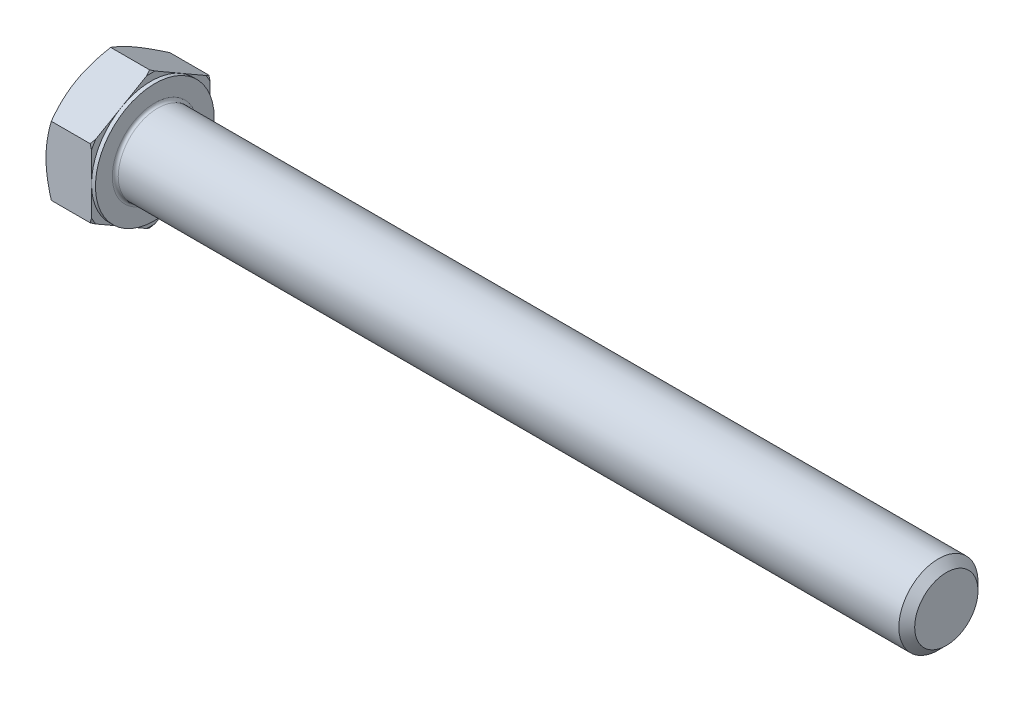
SolidWorks part; units mm, degrees
extrude "Base-Extrude" add sketch "Sketch1" along normal blind 10
sketch "Sketch1" plane through (0, 0, 0) normal (1, 0, 0) x (0, 0, -1)
  line L0 (12, 6.9282) -> (12, -6.9282)
  line L1 (-12, 6.9282) -> (-12, -6.9282)
  line L2 (12, -6.9282) -> (0, -13.8564)
  line L3 (0, -13.8564) -> (-12, -6.9282)
  line L4 (12, 6.9282) -> (0, 13.8564)
  line L5 (0, 13.8564) -> (-12, 6.9282)
revolve "Cut-Revolve1" cut sketch "Sketch3" angle 360 about L6
sketch "Sketch3" plane through (0, 0, 0) normal (0, 0, 1) x (1, 0, 0)
  line L0 (0, 12) -> (3.9585, 18.8564)
  line L1 (0, 13.8564) -> (0, 6.9282) construction
  line L2 (3.9585, 18.8564) -> (3.9585, 23.8564)
  line L3 (3.9585, 23.8564) -> (-10, 23.8564)
  line L4 (-10, 23.8564) -> (-10, 12)
  line L5 (-10, 12) -> (0, 12)
  line L6 (0, 0) -> (99.06, 0) construction
  line L7 (10, 13.8564) -> (0, 13.8564) construction
revolve "Boss-Revolve1" add sketch "Sketch2" angle 360 about L7
sketch "Sketch2" plane through (0, 0, 0) normal (0, 0, 1) x (1, 0, 0)
  line L0 (0, 6.9282) -> (0, -6.9282) construction
  line L1 (0, 0) -> (170, 0)
  line L2 (0, 0) -> (0, 8)
  line L3 (0, 8) -> (170, 8)
  line L4 (170, 0) -> (170, 6.268)
  line L5 (10, 13.8564) -> (10, 6.9282) construction
  line L7 (0, 0) -> (96.52, 0) construction
  line L8 (170, -6.268) -> (90.335, -8) construction
  line L9 (0, -8) -> (90.335, -8) construction
  line L10 (12, 15.24) -> (12, -1.27) construction
  line L11 (10, 15.24) -> (10, -1.27) construction
  line L12 (10, 6.9282) -> (10, -6.9282) construction
  line L14 (170, 8) -> (170, 6.268)
  dimension "l" = 160
  dimension "m" = 16
  dimension "Minor_dia" = 12.536
  dimension "p" = 2
  dimension "h" = 160
cosmetic thread "helix 1" parameters "Thread_length"=158, "Thread_minor"=12.536
ref_plane "front" through (0, 0, 0) normal (0, 0, 1) x (1, 0, 0)
ref_plane "top" through (0, 0, 0) normal (0, 1, 0) x (1, 0, 0)
ref_plane "right" through (0, 0, 0) normal (1, 0, 0) x (0, 0, -1)
sketch "Sketch5" plane through (0, 0, 0) normal (0, 0, 1) x (1, 0, 0)
  line L0 (10, 12) -> (6.0415, 18.8564)
  line L1 (10, 13.8564) -> (10, 6.9282) construction
  line L2 (6.0415, 18.8564) -> (6.0415, 23.8564)
  line L3 (6.0415, 23.8564) -> (16.0415, 23.8564)
  line L4 (16.0415, 23.8564) -> (16.0415, 12)
  line L5 (16.0415, 12) -> (10, 12)
  line L7 (10, 13.8564) -> (1.0718, 13.8564) construction
  line L8 (0, 0) -> (99.06, 0) construction
  line L9 (0, 0) -> (99.06, 0) construction
revolve "Cut-Revolve2" cut sketch "Sketch5" angle 360 about L8
sketch "Sketch4" plane through (0, 0, 0) normal (0, 0, 1) x (1, 0, 0)
  line L1 (10, 13.8564) -> (10, 6.9282) construction
  line L2 (10, 12) -> (9.2, 12)
  line L3 (10, 12) -> (10, 23.8564)
  line L4 (10, 23.8564) -> (9.2, 23.8564)
  line L5 (0, 0) -> (95.25, 0) construction
  line L6 (0, 0) -> (96.52, 0) construction
  line L7 (9.2, 12) -> (9.2, 23.8564)
  line L8 (8.9282, 13.8564) -> (1.0718, 13.8564) construction
revolve "Cut-Revolve3" cut sketch "Sketch4" angle 360 about L5
chamfer "Chamfer" distance 1.6 angle 45 1 edges at (170, 0, 8)
fillet "Fillet" radius 0.6 1 edges at (10, 0, -8)
sketch "Sketch6" plane through (0, 0, 0) normal (0, 0, 1) x (1, 0, 0)
  line L0 (11.6, -6.268) -> (10.6, -8)
  line L1 (11.6, -6.268) -> (12.5999, -8)
  line L2 (12.5999, -8) -> (12.5999, -10)
  line L3 (-3.175, 0) -> (5.1513, 0) construction
  line L5 (12.5999, -10) -> (10.6, -10)
  line L6 (10.6, -10) -> (10.6, -8)
  arc A0 (10.6, -8) -> (10, -8.6) centre (10.6, -8.6) ccw construction
revolve "Cut-Revolve4" [suppressed] cut sketch "Sketch6" angle 360 about L3
pattern_linear "LPattern1" [suppressed]
equation "\"D3@Sketch1\" = \"s@Sketch1\" / 2"
equation "\"D4@Sketch1\" = \"D3@Sketch1\""
equation "\"D5@Sketch1\" = \"D4@Sketch1\""
equation "\"D1@Sketch3\" = \"s@Sketch1\" / 2"
equation "\"D1@Sketch5\" = \"s@Sketch1\" / 2"
equation "\"Head_ch_ang@Sketch5\" = \"Head_ch_ang@Sketch3\""
equation "\"D1@Sketch4\" = \"s@Sketch1\""
equation "\"Diameter@Sketch6\" = \"m@Sketch2\""
equation "\"Overcut@Sketch6\" = \"m@Sketch2\" * 1.25"
equation "\"Minor_dia@Sketch2\" = \"m@Sketch2\"-\"p@Sketch2\" * 1.732"
equation "\"Thread_minor@helix 1\" = \"Minor_dia@Sketch2\""
equation "\"Thread_minor@Sketch6\" = \"Minor_dia@Sketch2\""
equation "\"D1@Chamfer\" = \"p@Sketch2\"*0.8"
equation "\"Thread_length@helix 1\" = \"l@Sketch2\" - \"p@Sketch2\""
equation "\"Num_threads@LPattern1\" = \"l@Sketch2\" / \"p@Sketch2\""
